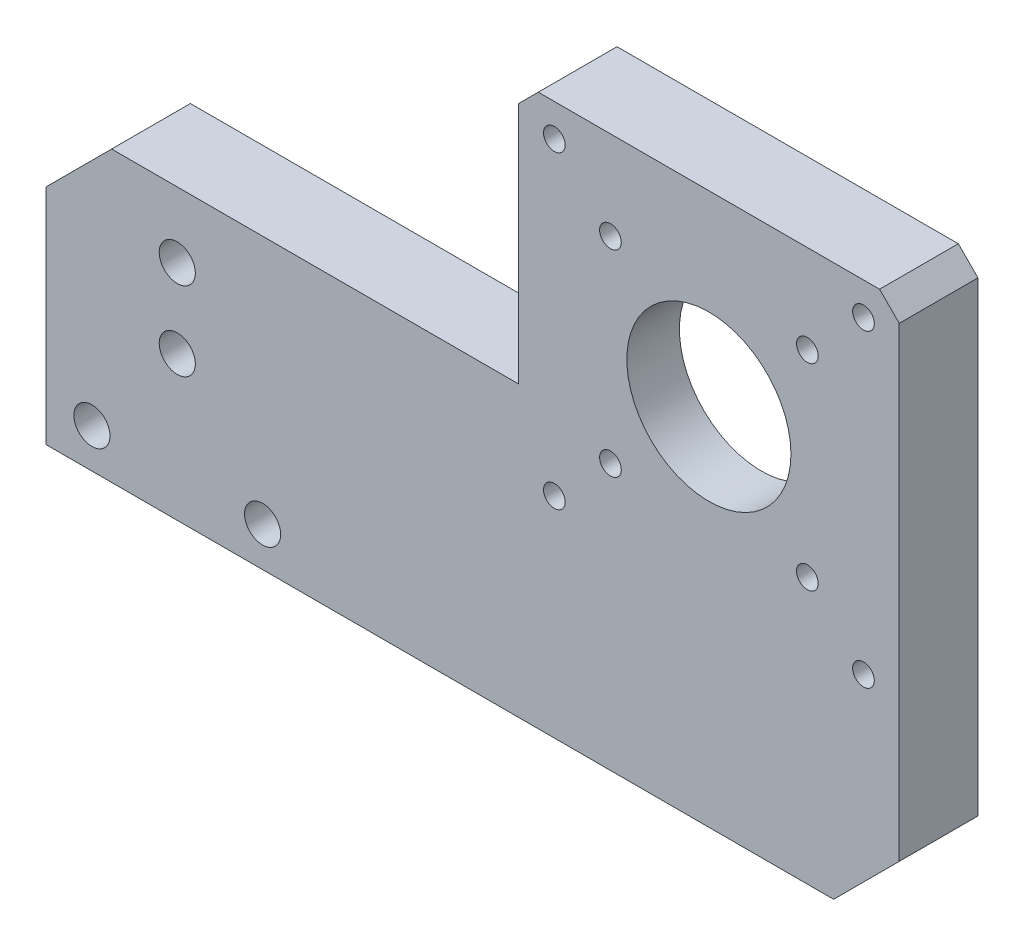
SolidWorks part; units mm, degrees
material "6063-T6"
ref_plane "前视" through (0, 0, 0) normal (0, 0, 1) x (1, 0, 0)
ref_plane "上视" through (0, 0, 0) normal (0, 1, 0) x (1, 0, 0)
ref_plane "右视" through (0, 0, 0) normal (1, 0, 0) x (0, 0, -1)
sketch "草图1" plane through (0, 0, 0) normal (0, 0, 1) x (1, 0, 0)
  line L2 (-29, -51.75) -> (29, -51.75)
  line L3 (-29, -51.75) -> (-29, 51.75)
  line L4 (-29, 51.75) -> (29, 51.75)
  line L5 (29, -51.75) -> (29, 51.75)
  line L6 (-29, -51.75) -> (29, 51.75) construction
  line L7 (-29, 51.75) -> (29, -51.75) construction
  point P0 (0, 0)
  dimension "D1" = 58
  dimension "D2" = 103.5
extrude "凸台-拉伸1" add sketch "草图1" along normal blind 12
sketch "草图2" plane through (0, 0, 0) normal (0, 0, -1) x (-1, 0, 0)
  line L0 (-29, 51.75) -> (29, 51.75) construction
  line L1 (23.55, -0.3) -> (-23.55, -0.3)
  line L2 (23.55, -0.3) -> (23.55, 46.8)
  line L3 (23.55, 46.8) -> (-23.55, 46.8)
  line L4 (-23.55, -0.3) -> (-23.55, 46.8)
  line L5 (23.55, -0.3) -> (-23.55, 46.8) construction
  line L6 (23.55, 46.8) -> (-23.55, -0.3) construction
  point P0 (0, 23.25)
  dimension "D1" = 47.1
  dimension "D2" = 28.5
hole_wizard "M4 螺纹孔1" positions "草图4" profile "草图3" tap size "M4" standard "Iso" end condition through all
sketch "草图4" plane through (0, 0, 0) normal (0, 0, -1) x (-1, 0, 0)
  point P0 (-23.55, 46.8)
  point P3 (23.55, 46.8)
  point P6 (23.55, -0.3)
  point P9 (-23.55, -0.3)
sketch "草图3" plane through (23.55, 46.8, 0) normal (1, 0, 0) x (0, 1, 0)
  line L0 (0, 0) -> (0, 12)
  line L1 (0, 12) -> (1.65, 12)
  line L2 (1.65, 12) -> (1.65, 0)
  line L5 (1.65, 0) -> (0, 0)
  line L11 (0, -6.35) -> (0, 107.95) construction
  dimension "通孔螺纹孔钻头直径" = 3.3
  dimension "通孔螺纹孔钻头深度" = 12
cosmetic thread "孔螺蚊线1" parameters "D2"=4
cosmetic thread "孔螺蚊线2" parameters "D2"=4
cosmetic thread "孔螺蚊线3" parameters "D2"=4
cosmetic thread "孔螺蚊线4" parameters "D2"=4
sketch "草图5" plane through (0, 0, 0) normal (0, 0, -1) x (-1, 0, 0)
  circle A0 centre (0, 23.25) radius 20
  dimension "D1" = 40
extrude "切除-拉伸1" cut sketch "草图5" against normal through all
sketch "草图6" plane through (0, -51.75, 0) normal (0, -1, 0) x (1, 0, 0)
  line L0 (29, 12) -> (29, 0) construction
  line L1 (-29, 0) -> (29, 0)
  line L2 (-29, 0) -> (-29, 58)
  line L3 (-29, 58) -> (29, 58)
  line L4 (29, 0) -> (29, 58)
  dimension "D1" = 58
extrude "凸台-拉伸2" add sketch "草图6" along normal blind 10
sketch "草图7" plane through (0, -51.75, 0) normal (0, -1, 0) x (1, 0, 0)
  line L0 (29, 58) -> (-29, 58) construction
  point P0 (-39, 52)
  point P1 (39, 52)
  dimension "D1" = 6
  dimension "D2" = 78
  dimension "D3" = 39
sketch "草图10" plane through (29, 0, 0) normal (1, 0, 0) x (0, 0, -1)
  line L0 (0, -61.75) -> (-58, -61.75) construction
  line L1 (-60, -51.75) -> (-12, -51.75)
  line L2 (-60, -51.75) -> (-60, -61.75)
  line L3 (-60, -61.75) -> (-12, -61.75)
  line L4 (-12, -51.75) -> (-12, -61.75)
  line L5 (-12, -51.75) -> (-12, 51.75) construction
  line L6 (-12, -51.75) -> (-58, -51.75) construction
  dimension "D1" = 48
extrude "切除-拉伸2" cut sketch "草图10" against normal blind 146
chamfer "倒角1" distance 3 angle 45 4 edges at (29, -61.75, 6) (-29, -61.75, 6) (-29, 51.75, 6) (29, 51.75, 6)
sketch "草图14" plane through (-29, 0, 0) normal (-1, 0, 0) x (0, 0, 1)
  line L0 (-30, -18.25) -> (43.8957, -18.25)
extrude "切除-拉伸5" cut sketch "草图14" against normal through all and the other way through all flip side to cut
sketch "草图15" plane through (0, 0, 0) normal (0, 0, -1) x (-1, 0, 0)
  line L1 (-29, -18.25) -> (101, -18.25)
  line L2 (-29, -18.25) -> (-29, -32.25)
  line L3 (-29, -32.25) -> (101, -32.25)
  line L4 (101, -18.25) -> (101, -32.25)
  dimension "D1" = 14
  dimension "D2" = 130
extrude "凸台-拉伸3" add sketch "草图15" against normal blind 12
sketch "草图16" plane through (0, 0, 12) normal (0, 0, 1) x (1, 0, 0)
  line L0 (29, -32.25) -> (-101, -32.25) construction
  line L1 (-101, -18.25) -> (-61, -18.25)
  line L2 (-101, -18.25) -> (-101, -32.25)
  line L3 (-101, -32.25) -> (-61, -32.25)
  line L4 (-61, -18.25) -> (-61, -32.25)
  dimension "D1" = 40
extrude "凸台-拉伸4" add sketch "草图16" along normal blind 60
sketch "草图17" plane through (-101, 0, 0) normal (-1, 0, 0) x (0, 0, 1)
  line L1 (72, -18.25) -> (84, -18.25)
  line L2 (72, -18.25) -> (72, -118.25)
  line L3 (72, -118.25) -> (84, -118.25)
  line L4 (84, -18.25) -> (84, -118.25)
  dimension "D1" = 12
  dimension "D2" = 100
extrude "凸台-拉伸5" add sketch "草图17" against normal up to vertex
sketch "草图18" plane through (0, 0, 0) normal (0, 0, -1) x (-1, 0, 0)
  line L0 (29, -18.25) -> (101, -18.25)
  line L2 (101, -18.25) -> (101, 11.75)
  line L4 (29, 11.75) -> (29, -18.25)
  line L5 (101, 11.75) -> (29, 11.75)
  dimension "D1" = 30
extrude "凸台-拉伸6" add sketch "草图18" against normal up to vertex
chamfer "倒角2" distance 10 angle 45 1 edges at (29, -32.25, 6)
sketch "草图19" plane through (0, 0, 12) normal (0, 0, 1) x (1, 0, 0)
  circle A0 centre (0, 23.25) radius 22.2484
  circle A1 centre (0, 23.25) radius 12.5
extrude "凸台-拉伸7" add sketch "草图19" against normal blind 8
sketch "草图20" plane through (0, -32.25, 0) normal (0, -1, 0) x (1, 0, 0)
  line L0 (-52.8445, 12) -> (-104.0072, 12)
  line L1 (19, 12) -> (-61, 12) construction
extrude "切除-拉伸6" cut sketch "草图20" along normal through all and the other way through all flip side to cut
hole_wizard "打孔尺寸根据六角头螺栓 C 级的类型0" positions "草图22" profile "草图21" counterbore size "M5" standard "Gb" end condition through all
sketch "草图22" plane through (0, 0, 0) normal (0, 0, -1) x (-1, 0, 0)
  line L0 (61, -32.25) -> (101, -32.25) construction
  line L1 (101, -32.25) -> (101, 11.75) construction
  point P0 (72.1485, 215.2425)
  point P1 (94, -26.25)
  point P3 (68, -26.25)
  point P10 (81, -10.25)
  point P12 (81, 1.75)
  dimension "D1" = 6
  dimension "D2" = 6
  dimension "D3" = 26
  dimension "D4" = 7
  dimension "D5" = 22
  dimension "D6" = 12
  dimension "D7" = 20
sketch "草图21" plane through (-72.1485, 215.2425, 0) normal (1, 0, 0) x (0, 1, 0)
  line L0 (0, 0) -> (0, 12)
  line L1 (0, 12) -> (2.75, 12)
  line L3 (2.75, 12) -> (2.75, 5.5)
  line L4 (2.75, 5.5) -> (5, 5.5)
  line L5 (5, 5.5) -> (5, 0)
  line L7 (5, 0) -> (0, 0)
  line L11 (0, -6.35) -> (0, 107.95) construction
  dimension "通孔孔直径" = 5.5
  dimension "通孔孔深度" = 12
  dimension "柱形沉头孔直径" = 10
  dimension "柱形沉头孔深度" = 5.5
chamfer "倒角3" distance 10 angle 45 1 edges at (-101, 11.75, 6)
hole_wizard "M4 螺纹孔2" positions "草图24" profile "草图23" tap size "M4" standard "Iso" end condition through all
sketch "草图24" plane through (0, 0, 12) normal (0, 0, 1) x (1, 0, 0)
  point P0 (15, 8.25)
  point P3 (-15, 8.25)
  point P6 (-15, 38.25)
  point P9 (15, 38.25)
sketch "草图23" plane through (15, 8.25, 12) normal (1, 0, 0) x (0, -1, 0)
  line L0 (0, 0) -> (0, 12)
  line L1 (0, 12) -> (1.65, 12)
  line L2 (1.65, 12) -> (1.65, 0)
  line L5 (1.65, 0) -> (0, 0)
  line L11 (0, -6.35) -> (0, 107.95) construction
  dimension "通孔螺纹孔钻头直径" = 3.3
  dimension "通孔螺纹孔钻头深度" = 12
cosmetic thread "孔螺蚊线9" parameters "D2"=4
cosmetic thread "孔螺蚊线10" parameters "D2"=4
cosmetic thread "孔螺蚊线11" parameters "D2"=4
cosmetic thread "孔螺蚊线12" parameters "D2"=4
